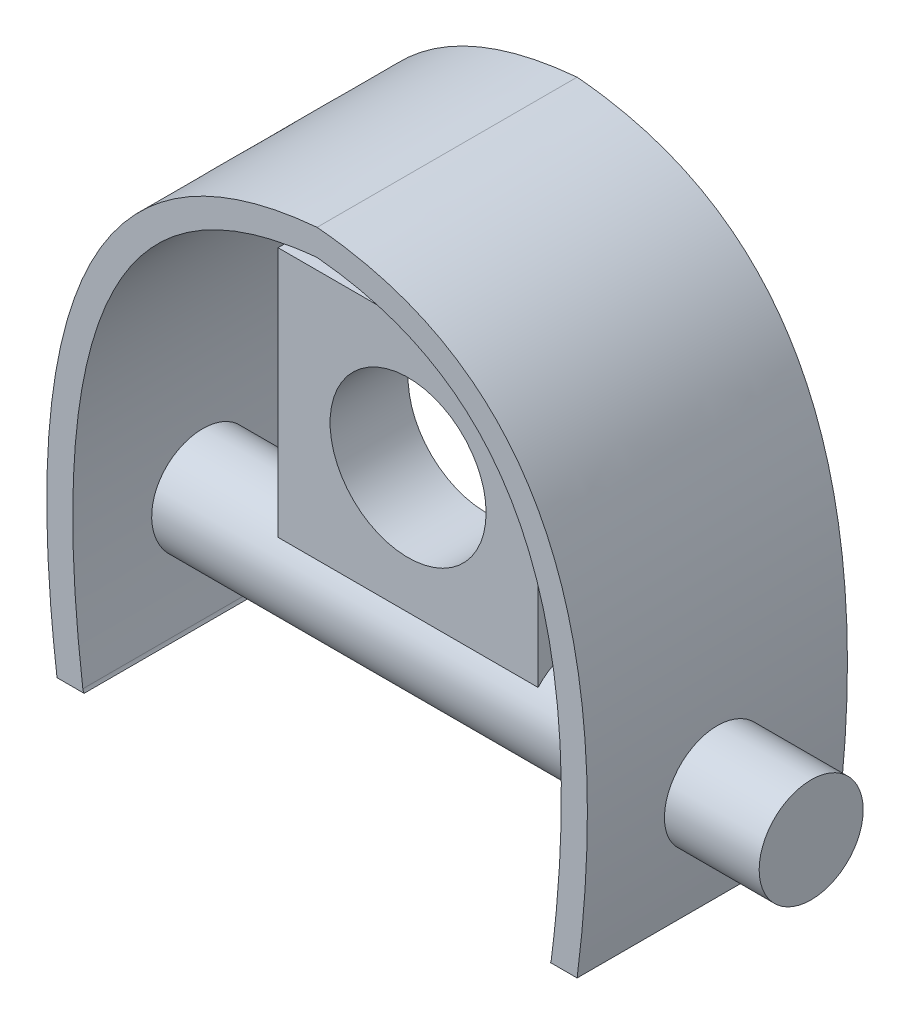
from build123d import *

# Parameters (mm, degrees)
BOSS_EXTRUDE1_DEPTH = 10
SKETCH3_R           = 2
BOSS_EXTRUDE2_DEPTH = 14
BOSS_EXTRUDE3_START = 10.5
SKETCH4_R           = 2
BOSS_EXTRUDE3_DEPTH = 10.5
SKETCH5_W           = 10
SKETCH5_H           = 10
BOSS_EXTRUDE4_DEPTH = 1.5
SKETCH6_R           = 3
CUT_EXTRUDE1_DEPTH  = 17


with BuildPart() as part:
    # Sketch1 → Boss-Extrude1 (new body)
    with BuildSketch(Plane.XY):
        with BuildLine():
            Line((10, 0), (8.973219811, 0))
            ThreePointArc((8.973219811, 0), (8.995129769, 0.062231167), (9.008087263, 0.12692172))
            add(Edge.make_bspline(
                [(0, 18.99589315), (0.463021411, 18.952514541), (1.410153528, 18.817218931), (3.070711392, 18.387284064), (4.862917757, 17.547866349), (6.569955551, 16.068587591), (7.897017979, 14.068512915), (8.836960927, 11.493329945), (9.27416213, 8.852445104), (9.404897772, 6.444073782), (9.391897127, 4.492140022), (9.286912223, 2.741425841), (9.147022016, 1.275055797), (9.056615507, 0.506177397), (9.008087263, 0.12692172)],
                knots=[0.003763747, 0.003763747, 0.003763747, 0.003763747, 0.066028513, 0.128293279, 0.252822811, 0.377352342, 0.501881874, 0.626411405, 0.750940937, 0.813205703, 0.875470468, 0.937735234, 0.968867617, 1, 1, 1, 1], degree=3))
            add(Edge.make_bspline(
                [(-9.008087263, 0.12692172), (-9.056615507, 0.506177397), (-9.147022016, 1.275055797), (-9.286912223, 2.741425841), (-9.391897127, 4.492140022), (-9.404897772, 6.444073782), (-9.27416213, 8.852445104), (-8.836960927, 11.493329945), (-7.897017979, 14.068512915), (-6.569955551, 16.068587591), (-4.862917757, 17.547866349), (-3.070711392, 18.387284064), (-1.410153528, 18.817218931), (-0.463021411, 18.952514541), (0, 18.99589315)],
                knots=[0.003763747, 0.003763747, 0.003763747, 0.003763747, 0.03489613, 0.066028513, 0.128293279, 0.190558045, 0.252822811, 0.377352342, 0.501881874, 0.626411405, 0.750940937, 0.875470468, 0.937735234, 1, 1, 1, 1], degree=3))
            ThreePointArc((-9.008087263, 0.12692172), (-8.991079354, 0.060388246), (-8.958380239, 0))
            Line((-8.958380239, 0), (-10, 0))
            add(Edge.make_bspline(
                [(0, 20), (-12.419499504, 18.908760189), (-10, 0)],
                knots=[0, 0, 0, 1, 1, 1], degree=2))
            add(Edge.make_bspline(
                [(0, 20), (12.419499504, 18.908760189), (10, 0)],
                knots=[0, 0, 0, 1, 1, 1], degree=2))
        make_face()
    extrude(amount=BOSS_EXTRUDE1_DEPTH)

    # Sketch3 → Boss-Extrude2 (add)
    with BuildSketch(Plane(origin=(0, 0, 0), x_dir=(0, 0, -1), z_dir=(1, 0, 0))):
        with Locations(Location((-5, 4.101905217, 0), (0, 0, 180))):
            Circle(SKETCH3_R)
    extrude(amount=BOSS_EXTRUDE2_DEPTH)

    # Sketch4 → Boss-Extrude3 (add)
    with BuildSketch(Plane.ZY.offset(BOSS_EXTRUDE3_START)):
        with Locations((5, 4.101905217)):
            Circle(SKETCH4_R)
    extrude(amount=-BOSS_EXTRUDE3_DEPTH)

    # Sketch5 → Boss-Extrude4 (add, symmetric)
    with BuildSketch(Plane.XY.offset(5)):
        with Locations((0, 10.070009498)):
            Rectangle(SKETCH5_W, SKETCH5_H)
    extrude(amount=BOSS_EXTRUDE4_DEPTH, both=True)

    # Sketch6 → Cut-Extrude1 (cut)
    with BuildSketch(Plane.XY.offset(6.5)):
        with Locations((0, 10.247395185)):
            Circle(SKETCH6_R)
    extrude(amount=-CUT_EXTRUDE1_DEPTH, mode=Mode.SUBTRACT)


solid = part.part
